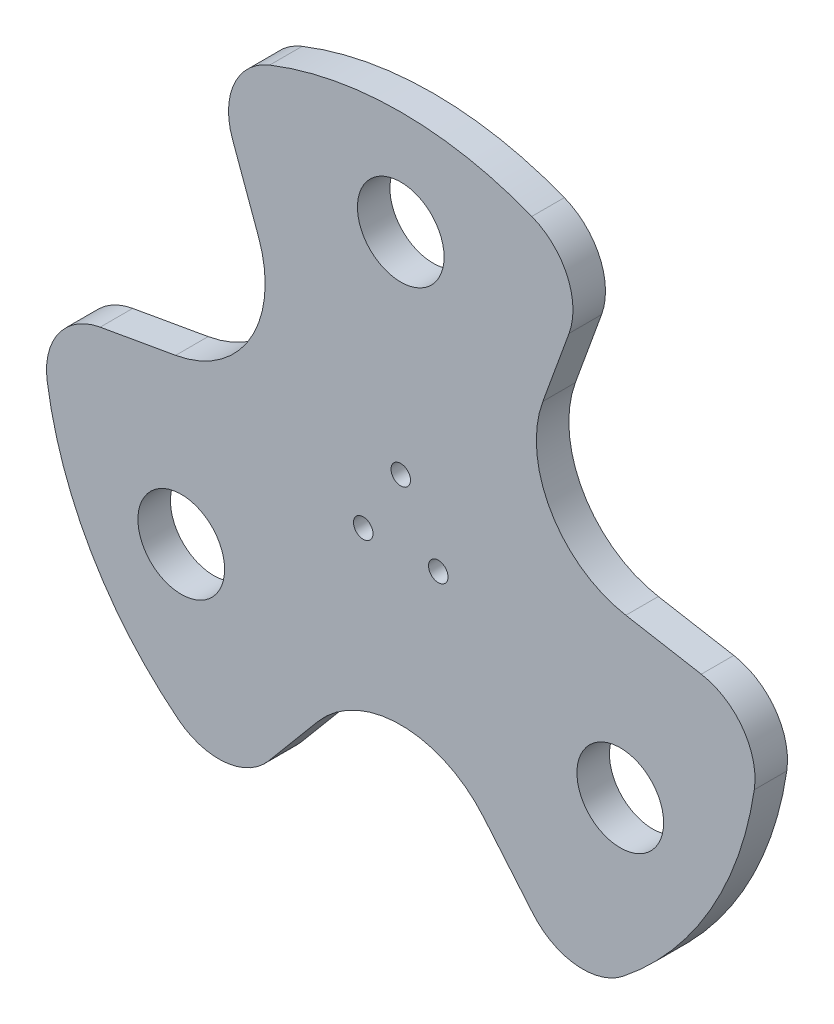
SolidWorks part; units mm, degrees
ref_plane "Front Plane" through (0, 0, 0) normal (0, 0, 1) x (1, 0, 0)
ref_plane "Top Plane" through (0, 0, 0) normal (0, 1, 0) x (1, 0, 0)
ref_plane "Right Plane" through (0, 0, 0) normal (1, 0, 0) x (0, 0, -1)
sketch "Sketch1" plane through (0, 0, 0) normal (0, 0, 1) x (1, 0, 0)
  circle A0 centre (0, 0) radius 165
  circle A1 centre (0, 117) radius 20
  circle A2 centre (101.325, -58.5) radius 20
  circle A3 centre (-101.325, -58.5) radius 20
  circle A5 centre (0, 30) radius 10.5 construction
  circle A6 centre (0, -30) radius 10.5 construction
  point P14 (0, 0)
  dimension "D1" = 330
  dimension "D3" = 40
  dimension "D6" = 21
  dimension "D2" = 117
  dimension "D5" = 60
  dimension "D7" = 30
  dimension "D4" = 3
extrude "Boss-Extrude1" add sketch "Sketch1" along normal blind 15
sketch "Sketch2" plane through (0, 0, 15) normal (0, 0, 1) x (1, 0, 0)
  line L0 (0, 0) -> (0, 130) construction
  line L1 (0, 0) -> (102.9043, 0) construction
  line L2 (-38.3022, 97.8606) -> (-169.9909, 254.801) construction
  line L3 (-169.9909, 254.801) -> (115.89, 190.3262) construction
  line L4 (115.89, 190.3262) -> (38.3022, 97.8606) construction
  line L14 (-38.3022, -97.8606) -> (-169.9909, -254.801)
  line L15 (-169.9909, -254.801) -> (115.89, -190.3262)
  line L16 (115.89, -190.3262) -> (38.3022, -97.8606)
  line L17 (-65.5987, 82.101) -> (-135.6687, 274.6169)
  line L18 (-135.6687, 274.6169) -> (-222.7723, -5.2006)
  line L19 (-222.7723, -5.2006) -> (-103.9009, 15.7596)
  line L20 (103.9009, 15.7596) -> (305.6596, -19.8159)
  line L21 (305.6596, -19.8159) -> (106.8823, 195.5268)
  line L22 (106.8823, 195.5268) -> (65.5987, 82.101)
  arc A0 (-38.3022, 97.8606) -> (38.3022, 97.8606) centre (0, 130) ccw construction
  arc A4 (-38.3022, -97.8606) -> (38.3022, -97.8606) centre (0, -130) cw
  arc A5 (-65.5987, 82.101) -> (-103.9009, 15.7596) centre (-112.5833, 65) cw
  arc A6 (103.9009, 15.7596) -> (65.5987, 82.101) centre (112.5833, 65) cw
  point P25 (0, 0)
  point P26 (0, 0)
  dimension "D3" = 100
  dimension "D1" = 90
  dimension "D2" = 130
  dimension "D4" = 40
  dimension "D6" = 293.0612
  dimension "D7" = 156.9404
  dimension "D5" = 3
extrude "Cut-Extrude1" cut sketch "Sketch2" against normal blind 30
fillet "Fillet1" radius 30 6 edges at (-78.1324, -145.3284, 7.5) (78.1324, -145.3284, 7.5) (164.9242, 4.9996, 7.5) (86.7919, 140.3288, 7.5) (-164.9242, 4.9996, 7.5) (-86.7919, 140.3288, 7.5)
sketch "Sketch3" plane through (0, 0, 15) normal (0, 0, 1) x (1, 0, 0)
  circle A0 centre (0, 20) radius 4.5
  circle A1 centre (17.3205, -10) radius 4.5
  circle A2 centre (-17.3205, -10) radius 4.5
  point P9 (0, 0)
  dimension "D1" = 9
  dimension "D2" = 20
  dimension "D3" = 3
extrude "Cut-Extrude2" cut sketch "Sketch3" against normal blind 20
